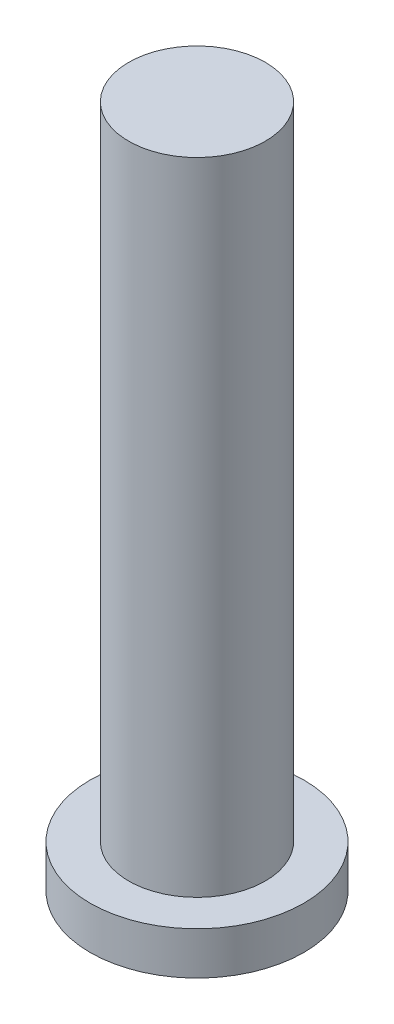
from build123d import *


with BuildPart() as part:
    # 草图1 → 旋转1 (revolve)
    with BuildSketch(Plane.XY, mode=Mode.PRIVATE) as revolve_1_sk:
        Polygon((0, 0), (4, 0), (4, -37.5), (6.25, -37.5), (6.25, -40), (0, -40), align=None)
    revolve(revolve_1_sk.sketch.rotate(Axis((0, -40, 0), (0, 1, 0)), 90), axis=Axis((0, -40, 0), (0, 1, 0)))


solid = part.part
